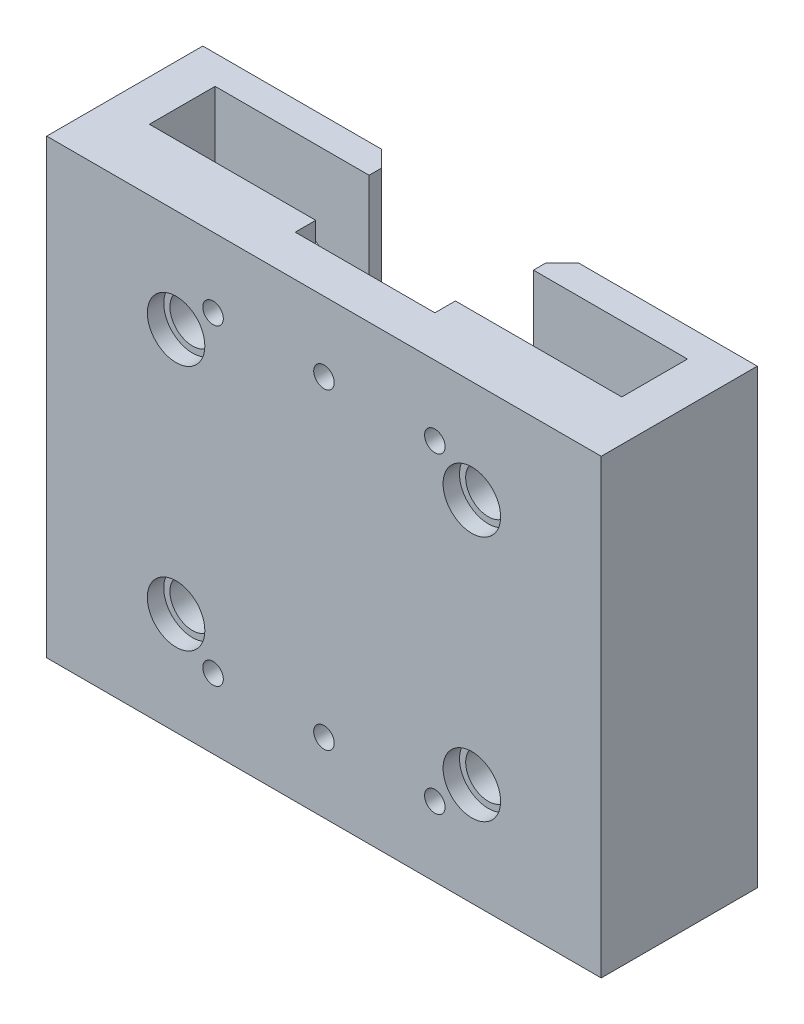
SolidWorks part; units mm, degrees
ref_plane "前视基准面" through (0, 0, 0) normal (0, 0, 1) x (1, 0, 0)
ref_plane "上视基准面" through (0, 0, 0) normal (0, 1, 0) x (1, 0, 0)
ref_plane "右视基准面" through (0, 0, 0) normal (1, 0, 0) x (0, 0, -1)
sketch "草图1" plane through (0, 0, 0) normal (0, 1, 0) x (1, 0, 0)
  line L1 (-67.5, -19) -> (67.5, -19)
  line L2 (-67.5, -19) -> (-67.5, 19)
  line L3 (-67.5, 19) -> (67.5, 19)
  line L4 (67.5, -19) -> (67.5, 19)
  line L5 (-67.5, -19) -> (67.5, 19) construction
  line L6 (-67.5, 19) -> (67.5, -19) construction
  point P0 (0, 0)
  dimension "D1" = 135
  dimension "D2" = 38
extrude "凸台-拉伸1" add sketch "草图1" along normal blind 110
sketch "草图3" plane through (0, 110, 0) normal (0, 1, 0) x (1, 0, 0)
  line L0 (0, 31.829) -> (0, -34.5331) construction
  line L2 (20, 19) -> (-20, 19)
  line L3 (67.5, 19) -> (-67.5, 19) construction
  line L4 (-20, 19) -> (-20, 12)
  line L5 (-20, 12) -> (-57.5, 12)
  line L6 (-57.5, 12) -> (-57.5, -4)
  line L7 (-57.5, -4) -> (-17, -4)
  line L8 (-17, -4) -> (-17, -9)
  line L9 (-17, -9) -> (17, -9)
  line L10 (17, -4) -> (17, -9)
  line L11 (57.5, -4) -> (17, -4)
  line L12 (57.5, 12) -> (57.5, -4)
  line L13 (20, 12) -> (57.5, 12)
  line L15 (20, 19) -> (20, 12)
  point P13 (0, -9)
  point P19 (0, 19)
  dimension "D1" = 40
  dimension "D2" = 34
  dimension "D3" = 5
  dimension "D4" = 16
  dimension "D5" = 7
  dimension "D6" = 115
extrude "切除-拉伸1" cut sketch "草图3" against normal through all
sketch "草图4" plane through (0, 0, -19) normal (0, 0, -1) x (-1, 0, 0)
  line L0 (-67.5, 110) -> (-20, 110) construction
  circle A0 centre (-36, 85) radius 11
  dimension "D1" = 22
  dimension "D2" = 36
  dimension "D3" = 25
extrude "切除-拉伸2" cut sketch "草图4" against normal blind 4
sketch "草图5" plane through (0, 0, -15) normal (0, 0, -1) x (-1, 0, 0)
  circle A0 centre (-36, 85) radius 5.5
  dimension "D1" = 11
extrude "切除-拉伸3" cut sketch "草图5" against normal through all
sketch "草图6" plane through (0, 0, 19) normal (0, 0, 1) x (1, 0, 0)
  circle A0 centre (36, 85) radius 7
  dimension "D1" = 14
extrude "切除-拉伸4" cut sketch "草图6" against normal blind 4
pattern_linear "阵列(线性)1" count 2 spacing 60 along (0, -1, 0) count 2 spacing 72 along (-1, 0, 0) of "切除-拉伸2", "切除-拉伸3", "切除-拉伸4"
hole_wizard "M6 螺纹孔1" positions "草图8" profile "草图7" tap size "M6" standard "GB"
sketch "草图8" plane through (0, 0, 19) normal (0, 0, 1) x (1, 0, 0)
  line L0 (-67.5, 0) -> (67.5, 0) construction
  point P0 (27, 93)
  dimension "D1" = 27
  dimension "D2" = 93
sketch "草图7" plane through (27, 93, 19) normal (1, 0, 0) x (0, -1, 0)
  line L0 (0, 0) -> (0, 13.4434)
  line L1 (0, 13.4434) -> (2.5, 12)
  line L2 (2.5, 12) -> (2.5, 0)
  line L5 (2.5, 0) -> (0, 0)
  line L10 (0, 13.4434) -> (-2.5, 12) construction
  line L11 (0, -6.35) -> (0, 107.95) construction
  dimension "螺纹孔钻头直径" = 5
  dimension "螺纹孔钻头深度" = 12
  dimension "导头角度" = 120
cosmetic thread "孔螺蚊线1" parameters "D1"=10, "D2"=6
pattern_linear "阵列(线性)2" count 3 spacing 27 along (-1, 0, 0) count 2 spacing 76 along (0, -1, 0) of "M6 螺纹孔1"
chamfer "倒角1" distance 4 angle 45 2 edges at (-20, 55, -19) (20, 55, -19)
